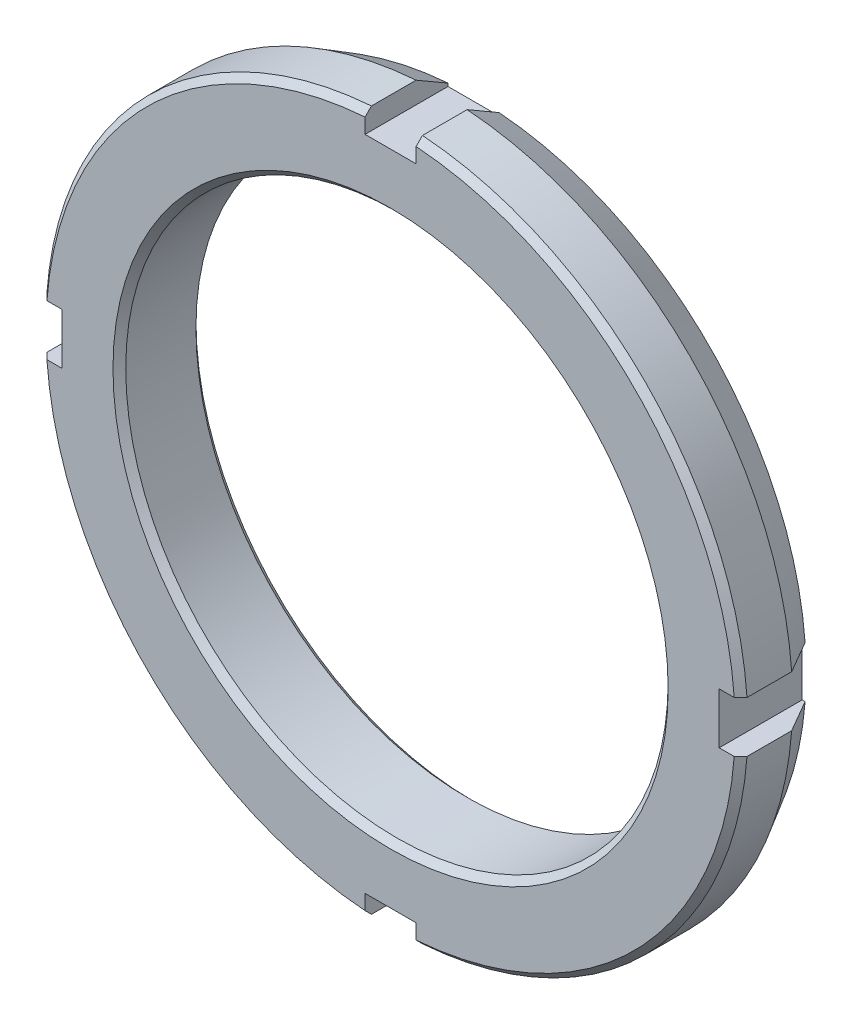
SolidWorks part; units mm, degrees
ref_plane "Front Plane" through (0, 0, 0) normal (0, 0, 1) x (1, 0, 0)
ref_plane "Top Plane" through (0, 0, 0) normal (0, 1, 0) x (1, 0, 0)
ref_plane "Right Plane" through (0, 0, 0) normal (1, 0, 0) x (0, 0, -1)
sketch "Sketch2" plane through (0, 0, 0) normal (0, 0, 1) x (1, 0, 0)
  circle A0 centre (0, 0) radius 110
  dimension "D1" = 220
extrude "Boss-Extrude1" add sketch "Sketch2" along normal blind 26
sketch "Sketch3" plane through (0, 0, 26) normal (0, 0, 1) x (1, 0, 0)
  line L2 (-8, 109.954) -> (-8, 103)
  line L3 (-109.954, -8) -> (-103, -8)
  line L4 (8, 109.954) -> (8, 103)
  line L5 (-109.954, 8) -> (-103, 8)
  line L6 (-103, 8) -> (-103, -8)
  line L8 (103, 8) -> (103, -8)
  line L9 (-8, 103) -> (8, 103)
  line L10 (103, 8) -> (109.954, 8)
  line L18 (103, -8) -> (109.954, -8)
  line L20 (-8, -103) -> (-8, -109.954)
  line L21 (8, -103) -> (8, -109.954)
  line L22 (-8, -103) -> (8, -103)
  arc A0 (8, 109.954) -> (-8, 109.954) centre (0, 0) ccw
  arc A1 (109.954, -8) -> (109.954, 8) centre (0, 0) ccw
  arc A2 (-8, -109.954) -> (8, -109.954) centre (0, 0) ccw
  arc A3 (-109.954, 8) -> (-109.954, -8) centre (0, 0) ccw
  circle A4 centre (0, 0) radius 110 construction
  point P5 (-8, 118.3124)
  point P6 (-8, -124.3705)
  point P7 (-123.1233, -8)
  point P8 (117.7778, -8)
  point P9 (8, 118.3124)
  point P10 (8, -124.3705)
  point P11 (-123.1233, 8)
  point P12 (117.7778, 8)
  point P13 (-103, 118.3124)
  point P14 (-103, -124.3705)
  point P15 (-123.1233, -103)
  point P16 (117.7778, -103)
  point P17 (103, 118.3124)
  point P18 (103, -124.3705)
  point P19 (-123.1233, 103)
  point P20 (117.7778, 103)
  dimension "D5" = 117.7778
  dimension "D1" = 110.2447
  dimension "D6" = 124.3705
  dimension "D9" = 123.1233
  dimension "D2" = 8
  dimension "D3" = 103
  dimension "D4" = 118.3124
extrude "Cut-Extrude1" cut sketch "Sketch3" against normal blind 26
chamfer "Chamfer1" distance 2 angle 45 4 edges at (77.7817, -77.7817, 26) (-77.7817, -77.7817, 26) (-77.7817, 77.7817, 26) (77.7817, 77.7817, 26)
chamfer "Chamfer2" distance 10 angle 30 4 edges at (-77.7817, -77.7817, 0) (77.7817, -77.7817, 0) (-77.7817, 77.7817, 0) (77.7817, 77.7817, 0)
sketch "Sketch4" plane through (0, 0, 0) normal (0, 0, -1) x (-1, 0, 0)
  circle A0 centre (0, 0) radius 85
  dimension "D1" = 170
extrude "Cut-Extrude2" cut sketch "Sketch4" against normal blind 26
sketch "Sketch5" plane through (0, 0, 0) normal (0, 0, -1) x (-1, 0, 0)
  circle A0 centre (0, 0) radius 86.5 construction
  dimension "D1" = 173
chamfer "Chamfer3" distance 2 angle 45 2 edges at (-85, 0, 26) (-85, 0, 0)
